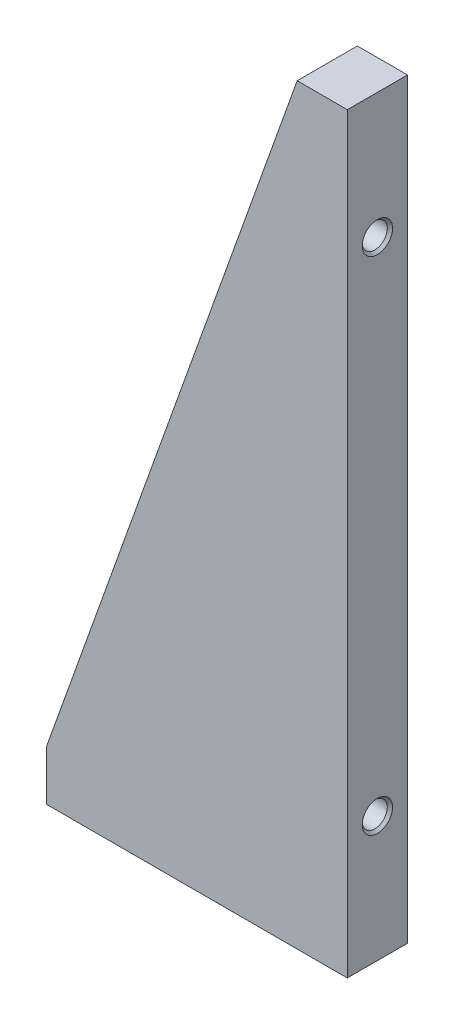
SolidWorks part; units mm, degrees
material "6061 合金"
ref_plane "前视基准面" through (0, 0, 0) normal (0, 0, 1) x (1, 0, 0)
ref_plane "上视基准面" through (0, 0, 0) normal (0, 1, 0) x (1, 0, 0)
ref_plane "右视基准面" through (0, 0, 0) normal (1, 0, 0) x (0, 0, -1)
sketch "草图1" plane through (0, 0, 0) normal (0, 0, 1) x (1, 0, 0)
  line L0 (0, 8.4564) -> (0, 18.4564)
  line L1 (0, 18.4564) -> (50, 158.4564)
  line L2 (50, 158.4564) -> (60, 158.4564)
  line L3 (60, 158.4564) -> (60, 8.4564)
  line L4 (60, 8.4564) -> (0, 8.4564)
  dimension "D1" = 60
  dimension "D2" = 150
  dimension "D3" = 10
  dimension "D4" = 10
extrude "凸台-拉伸1" add sketch "草图1" along normal blind 12
hole_wizard "M6 螺纹孔1" positions "草图2" profile "草图4" tap size "M6" standard "GB"
sketch "草图2" plane through (0, 8.4564, 0) normal (0, -1, 0) x (-1, 0, 0)
  line L0 (0, 0) -> (-60, 0) construction
  line L1 (0, -12) -> (0, 0) construction
  point P0 (-50, -6)
  point P3 (-10, -6)
  dimension "D1" = 6
  dimension "D2" = 10
  dimension "D3" = 40
sketch "草图4" plane through (50, 8.4564, 6) normal (1, 0, 0) x (0, 0, -1)
  line L0 (0, 0) -> (0, 16.5022)
  line L1 (0, 16.5022) -> (2.5, 15)
  line L2 (2.5, 15) -> (2.5, 0.525)
  line L3 (2.5, 0.525) -> (3.025, 0)
  line L5 (3.025, 0) -> (0, 0)
  line L6 (-2.5, 0.525) -> (-3.025, 0) construction
  line L10 (0, 16.5022) -> (-2.5, 15) construction
  line L11 (0, -6.35) -> (0, 107.95) construction
  dimension "螺纹孔钻头直径" = 5
  dimension "螺纹孔钻头深度" = 15
  dimension "近端锥形沉头孔直径" = 6.05
  dimension "近端锥形沉头孔角度" = 90
  dimension "导头角度" = 118
cosmetic thread "孔螺蚊线1"
cosmetic thread "孔螺蚊线2"
hole_wizard "M6 螺纹孔2" positions "草图5" profile "草图6" tap size "M6" standard "GB"
sketch "草图5" plane through (60, 0, 0) normal (1, 0, 0) x (0, 0, -1)
  line L0 (-12, 8.4564) -> (-12, 158.4564) construction
  line L1 (-12, 8.4564) -> (0, 8.4564) construction
  line L2 (-12, 158.4564) -> (0, 158.4564) construction
  point P0 (-6, 33.4564)
  point P2 (-6, 133.4564)
  dimension "D1" = 6
  dimension "D2" = 25
  dimension "D3" = 25
sketch "草图6" plane through (60, 33.4564, 6) normal (0, 1, 0) x (0, 0, -1)
  line L0 (0, 0) -> (0, 16.5022)
  line L1 (0, 16.5022) -> (2.5, 15)
  line L2 (2.5, 15) -> (2.5, 0.525)
  line L3 (2.5, 0.525) -> (3.025, 0)
  line L5 (3.025, 0) -> (0, 0)
  line L6 (-2.5, 0.525) -> (-3.025, 0) construction
  line L10 (0, 16.5022) -> (-2.5, 15) construction
  line L11 (0, -6.35) -> (0, 107.95) construction
  dimension "螺纹孔钻头直径" = 5
  dimension "螺纹孔钻头深度" = 15
  dimension "近端锥形沉头孔直径" = 6.05
  dimension "近端锥形沉头孔角度" = 90
  dimension "导头角度" = 118
cosmetic thread "孔螺蚊线3"
cosmetic thread "孔螺蚊线4"
